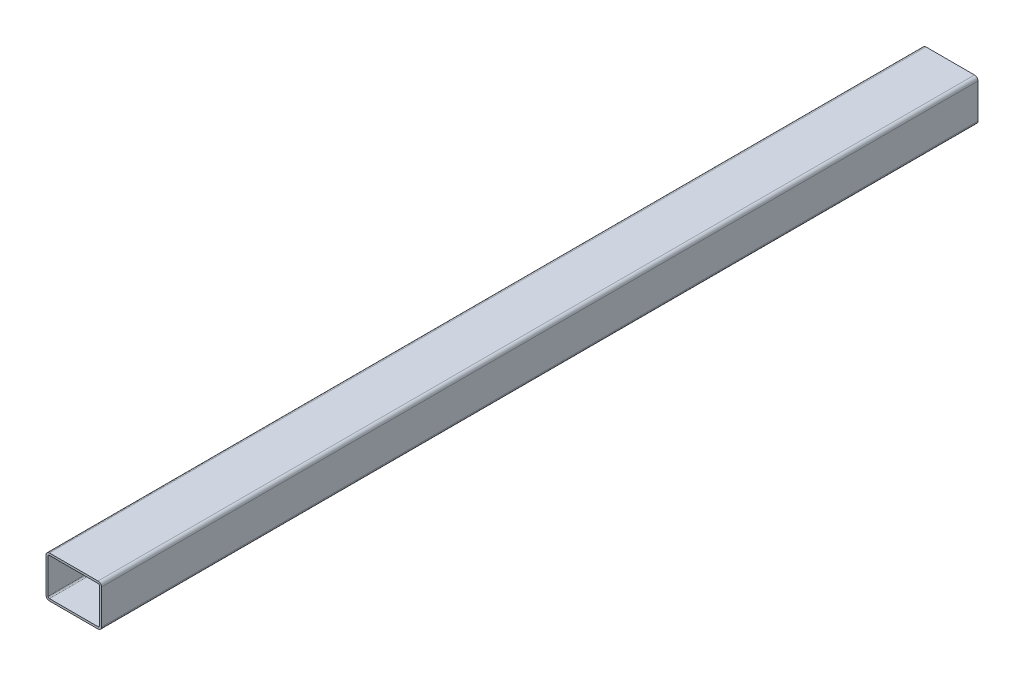
from build123d import *

# Parameters (mm, degrees)
SKETCH_1_W      = 80
SKETCH_1_H      = 60
EXTRUDE_1_DEPTH = 1264
FILLET_1_R      = 5
SHELL_1_T       = -3


with BuildPart() as part:
    # 草图1 → 凸台-拉伸1 (new body)
    with BuildSketch(Plane.XY):
        Rectangle(SKETCH_1_W, SKETCH_1_H)
    extrude(amount=EXTRUDE_1_DEPTH)

    # 圆角1
    fillet_1_edges = [part.edges().sort_by_distance(p)[0] for p in [
        (-40, 30, 632),
        (40, 30, 632),
        (40, -30, 632),
        (-40, -30, 632),
    ]]
    fillet(fillet_1_edges, radius=FILLET_1_R)

    # 抽壳1
    shell_1_openings = [part.faces().sort_by_distance(p)[0] for p in [
        (0, 0, 1264),
        (0, 0, 0),
    ]]
    offset(amount=SHELL_1_T, openings=shell_1_openings, kind=Kind.INTERSECTION)


solid = part.part
